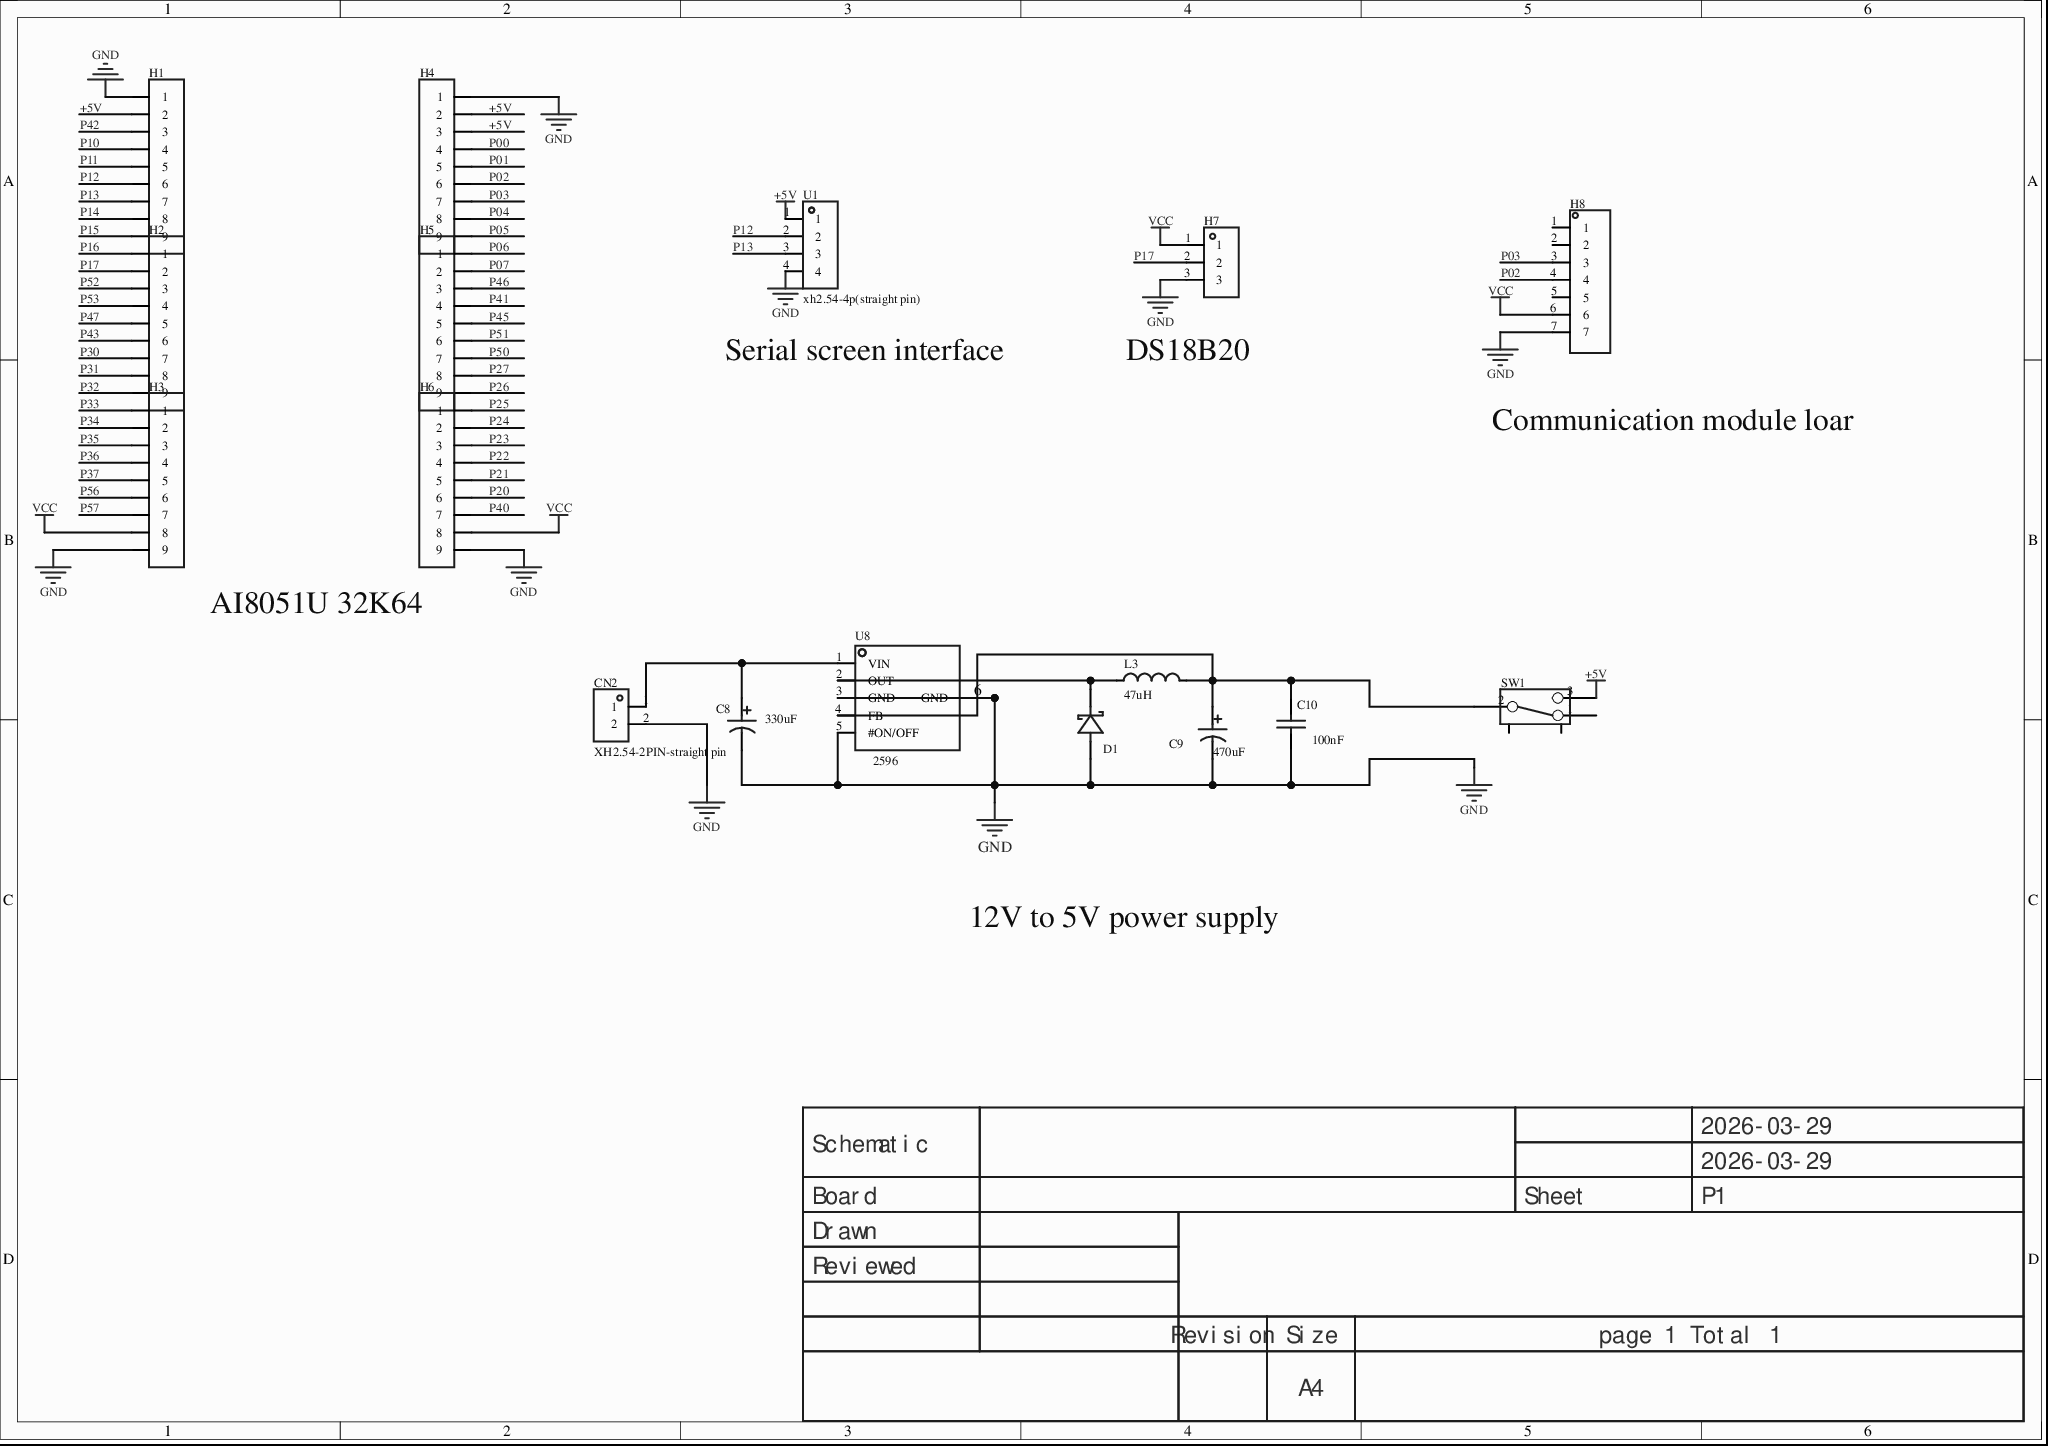
[diagram p0: MISC61480-3.schdoc]
# Altium project MISC61480-2.PrjPcb
1 sheet, 17 parts. Net scope: global (net labels, ports and power ports of the same name join across sheets).
Board file: MISC61480.pcbdoc

## Sheet MISC61480-3.schdoc
size 297 x 209 mm; Version: V1.0; @Project Name: MISC61480; @Update Date: 2026-03-29; @Create Date: 2026-03-29; @Board Name: MISC61480; @Create Time: 20:54:20; @Page Count: 1; @Page No: 1; @Schematic Name: MISC61480; @Update Time: 20:54:20; Size: A4

### Parts
C8  value 330uF  [CAP-SMD_BD8.0-L8.3-W8.3-RD]
C9  value 470uF  [CAP-SMD_BD8.0-L8.3-W8.3-RD]
C10  value 100nF  [C0805]
CN2  XH2.54-2PIN-straight pin  [CONN-TH_XH2.54-2P]
D1  (no value)  [SMA_L4.3-W2.6-LS5.2-RD]
H1  (no value)  [HDR-TH_9P-P2.54-V-F-1]
H2  (no value)  [HDR-TH_9P-P2.54-V-F-1]
H3  (no value)  [HDR-TH_9P-P2.54-V-F-1]
H4  (no value)  [HDR-TH_9P-P2.54-V-F-1]
H5  (no value)  [HDR-TH_9P-P2.54-V-F-1]
H6  (no value)  [HDR-TH_9P-P2.54-V-F-1]
H7  (no value)  [HDR-TH_3P-P2.54-V-F]
H8  (no value)  [HDR-TH_7P-P2.54-V-F]
L3  value 47uH  [IND-SMD_L7.0-W6.6]
SW1  (no value)  [拨动开关]
U1  xh2.54-4p(straight pin)  [CONN-TH_4P-P2.50-XH2.54-4P]
U8  LM2596S-5.0  [TO-263-5_L10.2-W8.9-P1.70-BR]  (value not drawn)

### Nets
+5V: H1.2 H4.2 H4.3 SW1.3 U1.1
GND: C8.2 C9.2 C10.2 CN2.2 D1.2(A) H1.1 H3.9 H4.1 H6.9 H7.3 H8.7 U1.4 U8.3(GND) U8.5(#ON/OFF) U8.6(GND)
VCC: H3.8 H6.8 H7.1 H8.6
P00: H4.4
P01: H4.5
P02: H4.6 H8.4
P03: H4.7 H8.3
P04: H4.8
P05: H4.9
P06: H5.1
P07: H5.2
P10: H1.4
P11: H1.5
P12: H1.6 U1.2
P13: H1.7 U1.3
P14: H1.8
P15: H1.9
P16: H2.1
P17: H2.2 H7.2
P20: H6.6
P21: H6.5
P22: H6.4
P23: H6.3
P24: H6.2
P25: H6.1
P26: H5.9
P27: H5.8
P30: H2.7
P31: H2.8
P32: H2.9
P33: H3.1
P34: H3.2
P35: H3.3
P36: H3.4
P37: H3.5
P40: H6.7
P41: H5.4
P42: H1.3
P43: H2.6
P45: H5.5
P46: H5.3
P47: H2.5
P50: H5.7
P51: H5.6
P52: H2.3
P53: H2.4
P56: H3.6
P57: H3.7
NetC8_1: C8.1 CN2.1 U8.1(VIN)
NetC9_1: C9.1 C10.1 L3.2 SW1.2 U8.4(FB)
NetD1_1: D1.1(K) L3.1 U8.2(OUT)

Not connected (* = marked no-connect by the designer): H8 1 2 5; SW1 1 4 5

### Notes on the sheet
- (near U1) Serial screen interface
- (near H7) DS18B20
- Communication module loar
- AI8051U 32K64
- 12V to 5V power supply
- 2026-03-29
- Schematic
- Board
- Sheet
- P1
- Drawn
- Reviewed
- Revision
- Size
- A4
- page 1 Total 1

### Library data of the parts
C8 C9 = CS1V221M-CRF10　: Capacitance: 220uF; tolerance: ±20%; rated voltage: 35V; body diameter: 8mm; body length: 10.5mm; ripple current: -; ESR: -; life: 2000hrs@105; operating temperature: -40~+105;; Manufacturer: ST(先科); Rated Voltage: 25V; 3D Model: b102f1362be24624a1b1334fec8dc7f4; 3D Model Transform: 354.33,326.81037,0,0,0,0,0,0,0; AddInBom: yes; Symbol: CS1V221M-CRF10; Device: CS1V221M-CRF10; Lifetime @ Temp: 2000hrs@105; Operating Temperature: -40~+105; Manufacturer Part: CS1V221M-CRF10; Supplier Footprint: SMD,8x10.5mm; JLCPCB Part Class: Extended Part; Datasheet: https://example.com/upload/public/pdf/source/20170325/1490427945143.pdf; Supplier: LCSC; Tolerance: ±20%; φD: 8mm; L: 10.5mm; Ripple Current: -; Equivalent Series Resistance(ESR): -; ConvertToPcb: yes; FootprintName: CAP-SMD_BD8.0-L8.3-W8.3-RD; ModelName: CAP-SMD_BD8.0-L8.3-W8.3-RD
  C8: Supplier Part: C97814
C10 = CL21B104KBCNNNC: Capacitance: 100nF; tolerance: ±10%; rated voltage: 50V; temperature coefficient: X7R;; Manufacturer: SAMSUNG(三星); 3D Model: 1ba041120af144c991958decab20d241; 3D Model Transform: 78.74,51.181,0,0,0,0,0,0.0005,0; AddInBom: yes; ModelName: C0805_L2.0-W1.3-H1.3; Symbol: CL21B104KBCNNNC; Device: CL21B104KBCNNNC; LCSC Part Name: 100nF ±10% 50V; Supplier Part: C1711; Manufacturer Part: CL21B104KBCNNNC; Supplier Footprint: 0805; JLCPCB Part Class: Extended Part; Datasheet: https://example.com/upload/public/pdf/source/20160103/1457707693305.pdf; Supplier: LCSC; Tolerance: ±10%; Voltage Rated: 50V; Temperature Coefficient: X7R; ConvertToPcb: yes; FootprintName: C0805
CN2 = XH2.54-2PIN-直针: AddInBom: yes; ModelId: c3cc11bd8b8748c1ae6bc231aac3a1ff0819f05c4eef4c71ace90d822a990e87; ModelTransform: 296.889,230.315,0,0,0,0,0,26.653,-137.795; Symbol: XH2.54-2PIN-straight pin; Device: XH2.54-2PIN-straight pin; LCSC Part Name: XH2.54-2PIN-直针; SupplierPart: C9900011425; ManufacturerPart: XH2.54-2PIN-直针; Supplier Footprint: XH2.54-2PIN; JLCPCB Part Class: Extended Part; Supplier: LCSC; ConvertToPcb: yes; FootprintName: CONN-TH_XH2.54-2P; ModelName: CONN-TH_XH2.54-2P
D1 = SS34_3: Manufacturer: TDD(台冠电子); Manufacturer Part: SS34; Symbol: SS34_C3032484; 3D Model: 7ed2c9d0a4a74bbdbba07ab4052caf5b; 3D Model Transform: 185.039,102.362,0,0,0,0,0,0,0; AddInBom: yes; Device: SS34_3; LCSC Part Name: SS34; Supplier Part: C3032484; Supplier Footprint: SMA; JLCPCB Part Class: Extended Part; Datasheet: https://example.com/upload/public/pdf/source/20220622/9D70D0693761B542BF6F533590093AA5.pdf; Supplier: LCSC; ConvertToPcb: yes; FootprintName: SMA_L4.3-W2.6-LS5.2-RD; ModelName: SMA_L4.3-W2.6-LS5.2-RD
H1-H6 = HDR-F_2.54_1x9P: Symbol: Header-Female-2.54_1x9; AddInBom: yes; ModelId: 3a7016416d904017ac5ead6cc0f14e9c0819f05c4eef4c71ace90d822a990e87; ModelName: HDR-TH_9P-P2.54-F-LI-1X9P; ModelTransform: 915.746,94.488,0,0,0,0,0,0,-125.984; Device: HDR-F_2.54_1x9P; ConvertToPcb: yes; FootprintName: HDR-TH_9P-P2.54-V-F-1; SupplierPart: C39576; Supplier Footprint: 插件
H7 = HDR-F_2.54_1x3P: Symbol: PM254V-11-03-H85; ConvertToPcb: yes; ModelId: f3b3cc5aae9641bf9e56fc160cef875b0819f05c4eef4c71ace90d822a990e87; ModelName: HDR2.54-F-LI-1X3P; ModelTransform: 299.9994,100,0,0,0,0,0,0,-118.11; Device: HDR-F_2.54_1x3P; AddInBom: yes; SupplierPart: C541850; Supplier Footprint: 插件; FootprintName: HDR-TH_3P-P2.54-V-F
H8 = HDR-F_2.54_1x7P: Symbol: 220S-1*7P H=8.5MM Ytype Gold-plated; ConvertToPcb: yes; ModelId: 4c31987253bc43b9b52c17be2a6d3f910819f05c4eef4c71ace90d822a990e87; ModelName: HDR-TH_7P-P2.54-F-LI-1X7P; ModelTransform: 715.7466,94.488,0,0,0,0,0,0,-118.11; Device: HDR-F_2.54_1x7P; AddInBom: yes; SupplierPart: C124418; Supplier Footprint: 插件; FootprintName: HDR-TH_7P-P2.54-V-F
L3 = CMLO0630H330MTT: Inductance: 33uH; tolerance: ±20%; DC resistance (DCR): 270mΩ;; Manufacturer: Cybermax(思博科技); 3D Model: 6860c29aec394a38a0f014af7f722a42; 3D Model Transform: 275.6,259.8,0,0,0,0,0,0,0; AddInBom: yes; ModelName: IND-SMD_L7.0-W6.6-H3.0; Symbol: CMLO0630H330MTT; Device: CMLO0630H330MTT; LCSC Part Name: 33uH ±20% 270mΩ; Manufacturer Part: CMLO0630H330MTT; Supplier Footprint: SMD; JLCPCB Part Class: Extended Part; Datasheet: https://example.com/upload/public/pdf/source/20201124/C961478_55C23F293F63DC1D2CF3D7AB16D0E182.pdf; Supplier: LCSC; Tolerance: ±20%; DC Resistance (DCR): 270mΩ; ConvertToPcb: yes; FootprintName: IND-SMD_L7.0-W6.6
SW1 = 拨动开关_正: Symbol: Toggle switch; Device: Toggle switch_pos; ConvertToPcb: yes; ModelId: 4321fe59a4074cbfb4989553f297c68f0819f05c4eef4c71ace90d822a990e87; ModelName: SW-TH_SS-12D02-VG4; ModelTransform: 370.09,208.7,472.35,0,0,0,0,0,-110; AddInBom: yes; Supplier Footprint: 插件; FootprintName: Toggle switch
U1 = xh2.54-4p(直针): AddInBom: yes; ModelId: c69236e4c0a047c6aeeeefc1552045f50819f05c4eef4c71ace90d822a990e87; ModelTransform: 492.125,228.346,0,180,0,0,0,-19.685,-137.795; Symbol: XH2.54-4P (straight pin); Device: xh2.54-4p(straight pin); LCSC Part Name: xh2.54-4p(直针); SupplierPart: C9900015350; ManufacturerPart: xh2.54-4p(直针); Supplier Footprint: CONN-TH_4P-P2.50-XH2.54-4P; JLCPCB Part Class: Extended Part; Supplier: LCSC; ConvertToPcb: yes; FootprintName: CONN-TH_4P-P2.50-XH2.54-4P; ModelName: CONN-TH_4P-P2.50-XH2.54-4P
U8 = LM2596S-5.0_C347421: Function type: step-down; output type: fixed; input voltage: 40V; output voltage: 5V; output current (max): 3A;; Manufacturer: UMW(广东友台半导体); Symbol: LM2596-TO263; Add into BOM: yes; 3D Model: 4e421a816a7f4d57b8710832ddea550a; 3D Model Transform: 401.574,560.17797,0,90,0,0,-45.276,0,0; Synchronous Rectification: No; Number of Outputs: 1; Topology: Buck; Switching Frequency: 150kHz; ModelName: TO-263-5-5P_L10.2-W8.7-H4.5-LS14.4-P1.70; Device: LM2596S-5.0_C347421; Convert to PCB: yes; LCSC Part Name: 降压型 输入40V 输出5V 3A; Supplier Part: C347421; Manufacturer Part: LM2596S-5.0; Supplier Footprint: TO-263-5; JLCPCB Part Class: Extended Part; Datasheet: https://example.com/upload/public/pdf/source/20211011/C7416AEF3194BD283261B8F2553C4145.pdf; Supplier: LCSC; Function: Step-down; Output Type: Fixed; Input Voltage: 40V; Output Voltage: 5V; Output Current (Max): 3A; Operating Temperature: -40℃~+125℃@(TA); FootprintName: TO-263-5_L10.2-W8.9-P1.70-BR